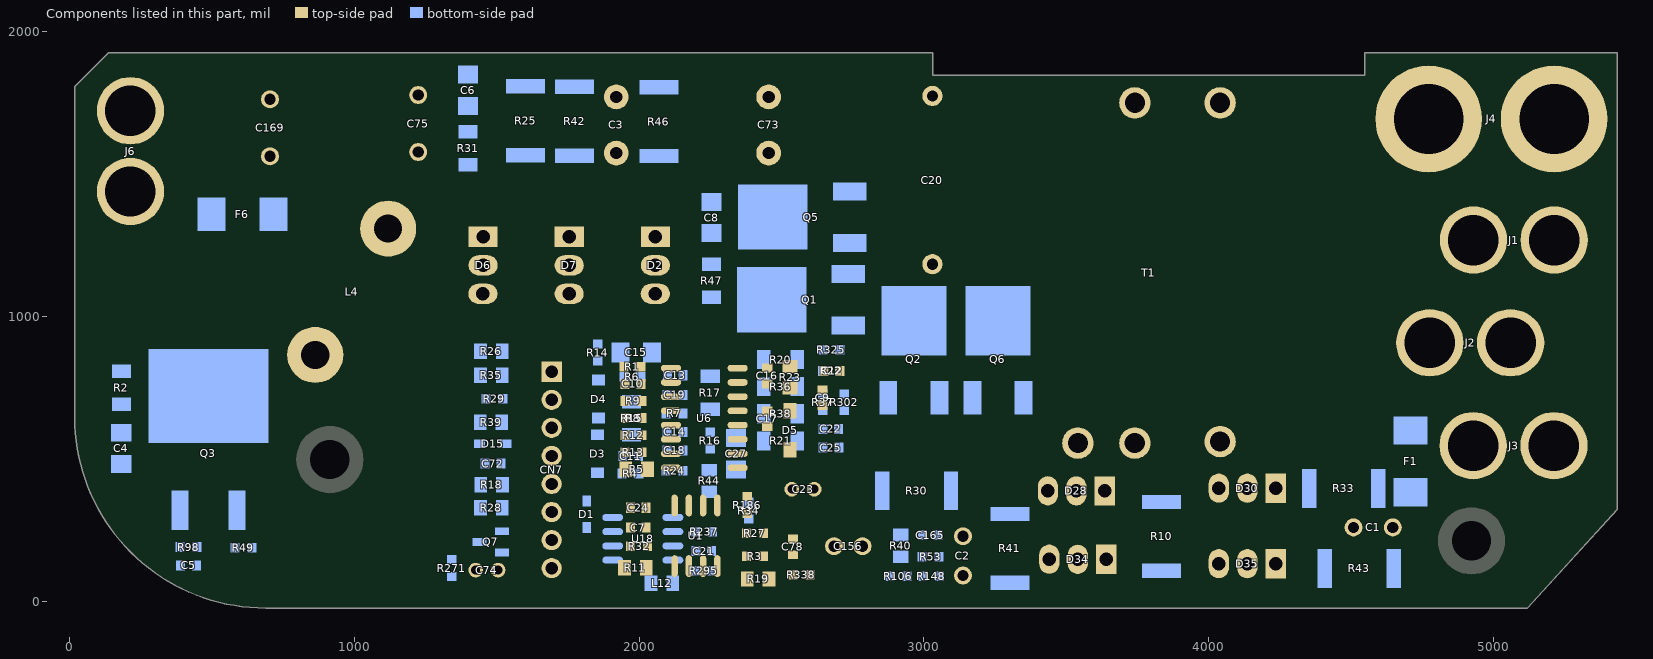
[diagram p0: the components of this part, seen from the top]
# Altium PCB MISC84449.PcbDoc (part 3 of 3)
Units mil, origin at the board's own origin, x right, y up, seen from the top; angles counter-clockwise.
Board outline 5413.39 x 1948.82 mil, 4 copper layers (Top Layer, GND02, PWR03, Bottom Layer); 124 components, 66 nets, 298 pads, 442 vias.

## Polygon pours and split planes (outlines as drawn) (continued)
BAT- on Top Layer "BottomLayer-No Net" (solid, remove dead copper, pour order 1000): 1796,1598 1796,1567 1796,1538 1807,1527 1837,1497 2313,1497 3038,1497 3063,1522 3104,1563 3104,1654 3104,1796 3104,1798 3088,1814 3084,1818 2990,1818 2855,1818 2840,1803 2837,1800 2837,1776 2837,1736 2819,1718 2751,1650 2492,1650 1822,1650 1803,1631 1796,1624 1796,1598
BAT- on Top Layer "BottomLayer-No Net" (solid, remove dead copper, pour order 1003): 5032,1731.08 5032,1694.35 5032,1545.33 5069,1506.5 5094,1480.26 5094,1278.77 5094,1103.51 4974,977.58 4942,944 4942,878.93 4942,842.2 5020,760.35 5094,682.69 5094,520.03 5094,166.37 5016,84.51 5005,72.97 4865,72.97 4790,72.97 4752,112.84 4720,146.43 4720,241.93 4720,282.85 4705,298.6 4702,301.74 4666,301.74 4617,301.74 4594,277.61 4588,271.31 4588,236.68 4588,105.5 4623,68.77 4679,10 4819,10 5038,10 5140,117.04 5368,356.31 5368,515.83 5368,1806.64 5313,1864.36 5300,1878 5253,1878 5140,1878 5090,1825.53 5032,1764.66 5032,1733.18
BAT- on GND02 "BottomLayer-No Net" (solid, remove dead copper, pour order 1001): 732,1081 537,1081 491,1035 455,999 455,865 455,392 572,275 612,235 771,235 1187,235 1308,356 1332,380 1332,728 1332,975 1251,1056 1226,1081 737,1081
BAT- on GND02 "BOTTOM-No Net" (solid, remove dead copper, pour order 1013): 5395,1925 5475,1845 5475,445 5040,10 3050,10 3035,25 3035,520 3025,530 2830,530 2790,570 2790,845 2660,975 1585,975 1335,725 1335,385 1185,235 730,235 695,270 695,1055 720,1080 1225,1080 1350,1205 1350,1350 1525,1525 1525,1910 3405,1910 3405,825 3425,805 4470,805 4615,950 4615,1665 4695,1745 4695,1900 4720,1925
GND on GND02 "BOTTOM-No Net" (solid, remove dead copper, pour order 1014): 1435,1580 1435,1920 1425,1930 85,1930 45,1890 5,1850 5,435 5,430 375,60 420,15 2880,15 2945,15 2955,25 2955,185 2955,430 2955,455 2945,465 2745,465 2720,465 2705,480 2695,490 2695,735 2695,820 2675,840 2610,905 1910,905 1640,905 1595,860 1415,680 1415,350 1415,345 1295,225 1225,155 940,155 570,155 515,210 385,340 385,860 385,1090 410,1115 505,1210 1075,1210 1215,1210 1260,1255 1260,1380 1260,1405 1435,1580
B+ on PWR03 "BottomLayer-No Net" (solid, remove dead copper, pour order 1003): 4570,1746 4570,1713.35 4570,778.97 4752,587.25 4792,545.12 4792,497.71 4792,452.42 4839,402.91 4856,385 4921,385 4992,385 5012,406.07 5058,454.52 5058,526.16 5058,576.72 4972,667.31 4902,741.05 4902,898.01 4902,1017.05 5015,1136.08 5047,1169.79 5047,1238.26 5047,1414.18 4999,1464.74 4979,1485.81 4979,1643.82 4979,1801.83 4923,1860.82 4901,1884 4820,1884 4600,1884 4586,1869.25 4570,1852.4 4570,1747.06
NetC1_1 on PWR03 "BottomLayer-No Net" (solid, remove dead copper, pour order 1002): 3035,234 3035,49 3072,12 3083,1 3173,1 4702,1 4720,19 4747,46 4747,165 4747,483 4506,724 4429,801 4219,801 3489,801 3453,765 3431,743 3431,703 3431,649 3373,591 3331,549 3331,481 3331,308 3306,283 3299,276 3192,276 3061,276 3042,257 3035,250 3035,235
BAT- on PWR03 "BottomLayer-No Net" (solid, remove dead copper, pour order 1004): 765,1081 675,1081 616,1022 580,986 425,986 208,986 153,931 109,887 109,807 109,438 334,213 409,138 700,138 1129,138 1236,245 1336,345 1336,429 1336,940 1239,1037 1195,1081 765,1081
BAT- on PWR03 "BottomLayer-No Net" (solid, remove dead copper, pour order 1003): 5034,1725.9 5034,1554.09 5081,1504.55 5095,1489.8 5095,1273.72 5095,1118.78 4997,1015.49 4948,963.84 4948,905.87 4948,840.52 5006,779.39 5099,681.37 5099,555.94 5099,438.94 5145,390.46 5172,362 5247,362 5327,362 5364,401 5407,446.32 5407,542.24 5407,1810.22 5356,1863.97 5337,1884 5275,1884 5128,1884 5095,1849.22 5030,1780.71 5030,1728.01
NetC3_1 on PWR03 "BOTTOM-No Net" (solid, remove dead copper, pour order 1017): 2375,1445 2565,1445 2575,1435 2575,980 2565,970 2370,970 2360,980 2360,1440 2365,1445 2375,1445
T1H on PWR03 "BOTTOM-No Net" (solid, remove dead copper, pour order 1018): 2875,1105 3310,1105 3315,1100 3315,915 3310,910 2870,910 2865,915 2865,1095 2875,1105
BAT- on PWR03 "BOTTOM-No Net" (solid, remove dead copper, pour order 1020): 3045,300 3290,300 3310,320 3310,580 3405,675 3405,1915 3395,1925 1540,1925 1525,1910 1525,1525 1355,1355 1355,1210 1225,1080 760,1080 700,1020 700,265 730,235 1170,235 1335,400 1335,730 1580,975 2660,975 2790,845 2790,570 2830,530 3025,530 3035,520 3035,310
GND on PWR03 "BOTTOM-No Net" (solid, remove dead copper, pour order 1021): 1440,1690 1440,1910 1420,1930 100,1930 15,1845 15,1085 35,1065 485,1065 600,1180 1185,1180 1245,1240 1245,1495
GND on PWR03 "BOTTOM-No Net" (solid, remove dead copper, pour order 1022): 1620,907 2580,907 2595,892 2665,822 2665,787 2665,482 2680,467 2890,467 2915,467 2925,457 2925,12 2915,2 1415,2 1400,17 1385,32 1385,672 1385,682 1410,707 1610,907 1620,907
T1H on Bottom Layer "BottomLayer-No Net" (solid, remove dead copper, pour order 1003): 2669,1319 2669,1299 2669,1226 2677,1218 2679,1216 2688,1216 2811,1216 2825,1202 2835,1192 2835,1179 2835,1034 2822,1021 2811,1010 2771,1010 2687,1010 2678,1001 2676,999 2676,983 2676,941 2680,937 2683,934 2691,934 2818,934 2830,922 2837,915 2837,904 2837,878 2846,869 2852,863 2864,863 3358,863 3376,881 3384,889 3384,912 3384,1341 3589,1546 3724,1546 3763,1546 3778,1561 3807,1590 3807,1718 3807,1793 3797,1803 3786,1814 3747,1814 3466,1814 3258,1606 3058,1406 2978,1406 2958,1406 2926,1374 2889,1337 2710,1337 2684,1337 2673,1326 2669,1322 2669,1319
NetC1_1 on Bottom Layer "BottomLayer-No Net" (solid, remove dead copper, pour order 1006): 4465.15,304 4465.15,244 4474.23,235 4515.6,194 4515.6,148 4515.6,98 4473.22,56 4454.05,37 4406.63,37 4028.24,37 3988.89,76 3965.68,99 3965.68,133 3965.68,180 3959.63,186 3943.49,202 3928.35,202 3743.7,202 3732.6,191 3720.49,179 3720.49,122 3720.49,92 3708.38,80 3697.29,69 3665,69 3412.74,69 3380.45,101 3338.07,143 3236.16,143 3131.23,143 3116.09,128 3106,118 3106,99 3106,60 3134.25,32 3144.34,22 3201.86,22 4712.36,22 4734.56,44 4784,93 4784,233 4784,423 4763.82,443 4730.52,476 4660.9,476 4544.86,476 4515.6,447 4465.15,397 4465.15,304
B+ on Bottom Layer "BottomLayer-No Net" (solid, remove dead copper, pour order 1005): 4569,1729.18 4569,582.28 4598,551.54 4599,550.48 4652,550.48 4768,550.48 4785,532.46 4801,515.5 4801,493.24 4801,445.54 4831,413.74 4860,383 4915,383 4994,383 5023,413.74 5062,455.08 5062,509.14 5062,619.38 4995,690.4 4900,791.09 4900,905.57 4900,998.85 5021,1127.11 5049,1156.79 5049,1246.89 5049,1346.53 4982,1417.55 4976,1423.91 4976,1627.42 4976,1800.2 4924,1855.32 4896,1885 4819,1885 4631,1885 4597,1848.96 4569,1819.28 4569,1729.18
NetD30_2 on Bottom Layer "BottomLayer-No Net" (solid, remove dead copper, pour order 1004): 4077,443 4077,317 4096,298 4111,283 4160,283 4394,283 4400,289 4412,301 4412,331 4412,496 4395,513 4392,516 4263,516 4097,516 4086,505 4077,496 4077,446
NetD6_2 on Bottom Layer "BottomLayer-No Net" (solid, remove dead copper, pour order 1016): 1357,1277 1357,1055 1391,1021 1422,990 1524,990 1576,990 1603,1017 1620,1034 1620,1116 1620,1381 1664,1425 1674,1435 1674,1528 1674,1576 1664,1586 1651,1599 1649,1599 1541,1599 1526,1584 1519,1577 1519,1543 1519,1500 1433,1414 1357,1338 1357,1277
NetD7_2 on Bottom Layer "BottomLayer-No Net" (solid, remove dead copper, pour order 1015): 1704,1560 1704,1429 1680,1405 1668,1393 1668,1313 1668,1033 1688,1013 1724,977 1809,977 1882,977 1901,996 1925,1020 1925,1071 1925,1399 1879,1445 1847,1477 1847,1556 1847,1581 1835,1593 1828,1600 1800,1600 1721,1600 1708,1587 1704,1583 1704,1561
NetD2_1 on Bottom Layer "BottomLayer-No Net" (solid, remove dead copper, pour order 1014): 144,842 144,790 148,786 152,782 174,782 249,782 261,770 273,758 273,739 273,566 280,559 282,557 301,557 703,557 714,568 827,681 927,681 1009,681 1047,719 1064,736 1064,784 1064,971 1037,998 988,1047 852,1047 710,1047 678,1015 631,968 472,968 175,968 162,955 144,937 144,842
BAT- on Bottom Layer "BottomLayer-No Net" (solid, remove dead copper, pour order 1013): 140,497 140,367 329,178 337,170 389,170 397,170 405,178 409,182 409,201 409,234 422,247 436,261 436,302 436,389 456,409 470,423 555,423 631,423 660,394 664,390 664,311 664,278 682,260 687,255 709,255 808,255 820,267 828,275 828,291 828,360 794,394 665,523 557,523 151,523 144,516 140,512 140,497
NetD34_2 on Bottom Layer "BottomLayer-No Net" (solid, remove dead copper, pour order 1012): 3228,319 3228,312 3228,273 3241,260 3266,235 3335,235 3445,235 3478,202 3485,195 3485,166 3485,120 3501,104 3515,90 3537,90 3569,90 3582,103 3592,113 3592,146 3592,219 3571,240 3563,248 3548,248 3526,248 3476,298 3464,310 3447,310 3411,310 3384,337 3372,349 3322,349 3249,349 3231,331 3228,328 3228,320
BAT- on Bottom Layer "BottomLayer-No Net" (solid, remove dead copper, pour order 1011): 2799,747 2799,580 2815,564 2820,559 2861,559 2995,559 3011,543 3054,500 3054,377 3054,320 3061,313 3063,311 3082,311 3127,311 3132,316 3135,319 3135,334 3135,338 3141,344 3146,349 3190,349 3214,349 3222,357 3223,358 3223,459 3223,487 3246,510 3253,517 3253,583 3253,782 3241,794 3234,801 3204,801 3136,801 3133,798 3128,793 3128,785 3128,634 3118,624 3114,620 3053,620 2977,620 2959,638 2953,644 2953,685 2953,794 2947,800 2946,801 2935,801 2818,801 2815,798 2799,782 2799,747
BAT- on Bottom Layer "BottomLayer-No Net" (solid, remove dead copper, pour order 1009): 5032,1737.69 5032,1560.99 5079,1513.54 5097,1495.36 5097,1251.02 5097,1134.9 4961,997.58 4943,979.41 4943,899.64 4943,879.45 5045,776.46 5102,718.91 5102,491.73 5102,463.46 5127,438.21 5149,416 5193,416 5321,416 5357,452.35 5369,464.47 5369,478.6 5369,1804.33 5309,1864.91 5300,1874 5252,1874 5138,1874 5049,1784.14 5032,1766.97 5032,1738.7
NetD35_2 on Bottom Layer "BottomLayer-No Net" (solid, remove dead copper, pour order 1008): 4081,165.4 4081,88.08 4093,75.71 4116,52 4183,52 4432,52 4440,60.25 4452,72.62 4452,115.92 4452,208.7 4442,219.01 4410,252 4365,252 4112,252 4097,236.54 4083,222.1 4083,166.43
NetD28_2 on Bottom Layer "BottomLayer-No Net" (solid, remove dead copper, pour order 1006): 3493,422 3493,396 3493,308 3518,283 3537,264 3589,264 3888,264 3908,284 3926,302 3926,347 3926,460 3906,480 3895,491 3845,491 3518,491 3499,472 3494,467 3494,423
no net on Bottom Layer "BOTTOM-No Net" (solid, remove dead copper, pour order 1017): 2405,1465 2525,1465 2535,1455 2535,1315 2525,1305 2400,1305 2395,1310 2395,1455
PV+ on Bottom Layer "BOTTOM-No Net" (solid, remove dead copper, pour order 1023): 175,1545 540,1545 560,1525 560,1060 535,1035 95,1035 70,1060 70,1530 80,1540 85,1545 175,1545
PV-OVP on Bottom Layer "BOTTOM-No Net" (solid, remove dead copper, pour order 1025): 685,1680 635,1630 635,1150 670,1115 1165,1115 1305,1255 1305,1650 1275,1680
GND on Bottom Layer "BOTTOM-No Net" (solid, remove dead copper, pour order 1026): 175,1610 455,1610 550,1610 565,1625 565,1705 575,1715 765,1715 1315,1715 1330,1730 1330,1805 1345,1820 1350,1825 1445,1825 1455,1825 1460,1830 1460,1905 1450,1915 1440,1925 175,1925 105,1925 80,1900 30,1850 30,1700 30,1620 35,1615 40,1610 175,1610
NetC3_1 on Bottom Layer "BOTTOM-No Net" (solid, remove dead copper, pour order 1027): 2930,1905 2950,1885 2950,1690 2930,1670 2610,1670 2590,1650 2590,950 2585,945 2345,945 2335,955 2335,1650 2310,1675 2190,1675 2145,1720 1530,1720 1520,1730 1520,1895 1530,1905
NetD2_2 on Bottom Layer "BOTTOM-No Net" (solid, remove dead copper, pour order 1028): 1987,1631 2147,1631 2162,1616 2167,1611 2167,1476 2167,1456 2187,1436 2197,1426 2197,1206 2197,976 2192,971 2187,966 2022,966 1972,966 1962,976 1962,1026 1962,1626 1967,1631 1987,1631
GND on Bottom Layer "BOTTOM-No Net" (solid, remove dead copper, pour order 1039): 2595,490 2865,490 2880,475 2880,285 2860,265 2850,255 2840,245 2840,190 2840,160 2825,145 2510,145 2480,175 2480,470 2490,480 2500,490 2595,490

## Keep-outs
Keep-Out Layer:
  the board outline again, w6

## Other copper
Top Layer:
  rectangle net NetD2_1: 1361,1248 1546,1308
  rectangle net NetD2_1: 1411,1273 1486,1348
  rectangle net NetD2_1: 1713.5,1273 1788.5,1348
  rectangle net NetD2_1: 1663.5,1248 1848.5,1308
  rectangle net NetD2_1: 2023,1275 2098,1350
  rectangle net NetD2_1: 1973,1250 2148,1310
  rectangle net NetD2_1: 1410.61,1008 1485.61,1083
  rectangle net NetD2_1: 1360.61,1048 1545.61,1108
  rectangle net NetD2_1: 1723.11,998 1798.11,1073
  rectangle net NetD2_1: 1673.11,1038 1858.11,1098
  rectangle net NetD2_1: 2022.61,1010 2097.61,1085
  rectangle net NetD2_1: 1972.61,1050 2157.61,1110
  rectangle net LLC_I: 3150,1220 3300,1275
  rectangle net LLC_I: 3195,1185 3255,1315
  rectangle net GND: 55,1630 405,1810
  rectangle net GND: 120,1720 300,1870
  rectangle net GND: 640,1740 770,1785
  rectangle net GND: 680,1705 725,1825
  rectangle net GND: 1160,1755 1290,1800
  rectangle net GND: 1200,1710 1250,1845
  rectangle net +12V: 2475,510 2530,555
  rectangle net +12V: 2510,475 2545,515
  rectangle net +12V: 2484.6,380 2535,411.4
  rectangle net +12V: 2625,170 2690,215
  rectangle net +12V: 2660,194.99 2684.62,250
GND02:
  rectangle net GND: 1610,287.64 1735,343.64
  rectangle net BAT-: 5141,1113.64 5277,1425.64
  rectangle net BAT-: 5098,402 5293,697
  rectangle net GND: 130,1585 295,1870
  rectangle net GND: 65,1670 370,1790
PWR03:
  rectangle net GND: 1610,287.64 1735,343.64
  rectangle net BAT-: 2720,1535 2870,1600
  rectangle net BAT-: 2765,1495 2820,1640
  rectangle net BAT-: 2205,1535 2355,1595
  rectangle net BAT-: 2260,1485 2305,1635
  rectangle net GND: 65,1670 370,1790
  rectangle net GND: 130,1585 295,1870
Bottom Layer:
  rectangle net PV+: 460,1240 540,1465
  rectangle net PV+: 420,1310 500,1405
  rectangle net PV+: 70,1345 400,1521.43
  rectangle net PV+: 140,1265 290,1420
  rectangle net PV-OVP: 645,1540 780,1585
  rectangle net PV-OVP: 680,1500 730,1620
  rectangle net PV-OVP: 1160,1552.55 1280,1603.52
  rectangle net PV-OVP: 1195,1518.52 1240,1638.52
  rectangle net PV-OVP: 640,1315 815,1405
  rectangle net PV-OVP: 680,1260 755,1460
  rectangle net NetD6_2: 1366,1138 1536,1208
  rectangle net NetD7_2: 1666,1148 1836,1208
  rectangle net GND: 640,1735 775,1785
  rectangle net GND: 680,1760 730,1820
  rectangle net GND: 70,1635 360,1805
  rectangle net GND: 125,1710 305,1870
  rectangle net GND: 1150,1755 1300,1800
  rectangle net GND: 1200,1720 1250,1835
  rectangle net GND: 1380,1853.27 1425,1901.73
  rectangle net GND: 1335,1825 1395,1875
  rectangle net NetC3_1: 1525,1745 2145,1875
  rectangle net NetC3_1: 2335,955 2590,1495
  rectangle net NetD2_2: 1975.5,1150 2145.5,1210
  rectangle net T1H: 2670,1215 2845,1329.42
  rectangle net BAT-: 2818.73,645 2945,800
  rectangle net BAT-: 3135,645 3235,800
  rectangle net GND: 2775,280 2880,482.65
  rectangle net GND: 2760,180 2810,255
  rectangle net GND: 2600,330 2635,455
  rectangle net GND: 2620,375 2675,415

## Silkscreen, mask and mechanical layers (free items; w line width, h text height)
Top Overlay:
  lines w5: 1912.3,770.48 1922.01,770.48
Bottom Overlay:
  lines w5: 1916.6,510 1900,510 1900,330 2045,330 2045,510 2026.65,510 ; 2072.7,752.3 2072.7,827.7 2102.7,827.7 ; 2181.65,725.48 2197.3,725.48
Bottom Solder:
  lines w39.37: 1589,1216 1589,1424 ; 1893,1215 1893,1427 ; 1993,1214 1993,1426 ; 3471,307 3622,307 ; 3664,367 3857,367 ; 4274,377 4479,377 ; 4275,60 4460,60 ; 4275,300 4480,300 4505,275 4505,230
  lines w78.74: 5100,355 5100,445 5190,535
Mechanical 12:
  circle w6: c4921.42,214.1 r68.9
  circle w6: c915.52,499.54 r68.9
  lines w3.94: 59.22,1257.41 374.18,1257.41 374.18,1887.33 59.22,1887.33 59.22,1257.41 ; 4763.94,430.64 4763.94,1808.59 5393.87,1808.59 5393.87,430.64 4763.94,430.64
Mechanical 15:
  lines w0.1: 1199.56,833.07 1199.58,833.09 ; 2954.32,2313.19 2954.34,2313.21 ; 4269.47,623.41 4269.49,623.39
  lines w1.97: 1866.64,-1700.81 1866.64,4199.88 ; 3523.95,-1919.91 3523.95,3731.45